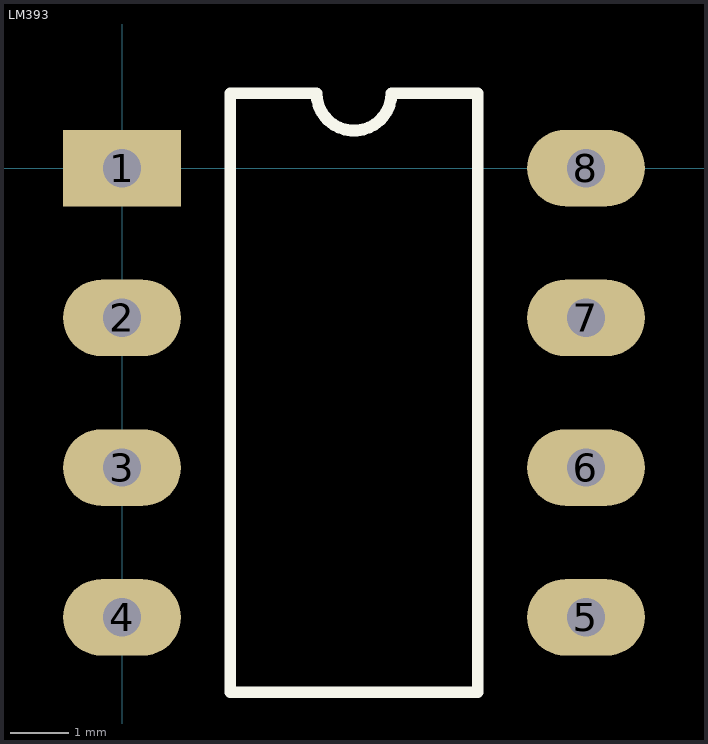
[diagram p0: the footprints below, top view; thin cyan lines are the x and y axes]
# Altium footprint library MISC86340-11.PcbLib: 3 footprints
Each footprint in its own frame and in the unit in brackets; x right, y up, seen from the top. Pads: shape width x height; smd on the part's side, far side on the other; paste and mask are expansions set on the pad; w line width, h text height; cw(c..) or ccw(c..) is an arc to the next point about the centre after c.

## LC-DIP-8 [mm]

## LM393 [mm]
pads (8):
  rect 2x1.3 hole 0.65: 1(0,0)
  oval 2x1.3 hole 0.65: 2(0,-2.54) 3(0,-5.08) 4(0,-7.62) 5(7.87,-7.62) 6(7.87,-5.08) 7(7.87,-2.54) 8(7.87,0)
Top Overlay:
  lines w0.2: 1.835,-8.89 1.835,1.27 3.3,1.27 ccw(c3.935,1.27) 4.57,1.27 6.035,1.27 6.035,-8.89 1.835,-8.89

## PCBComponent_1 [mm]